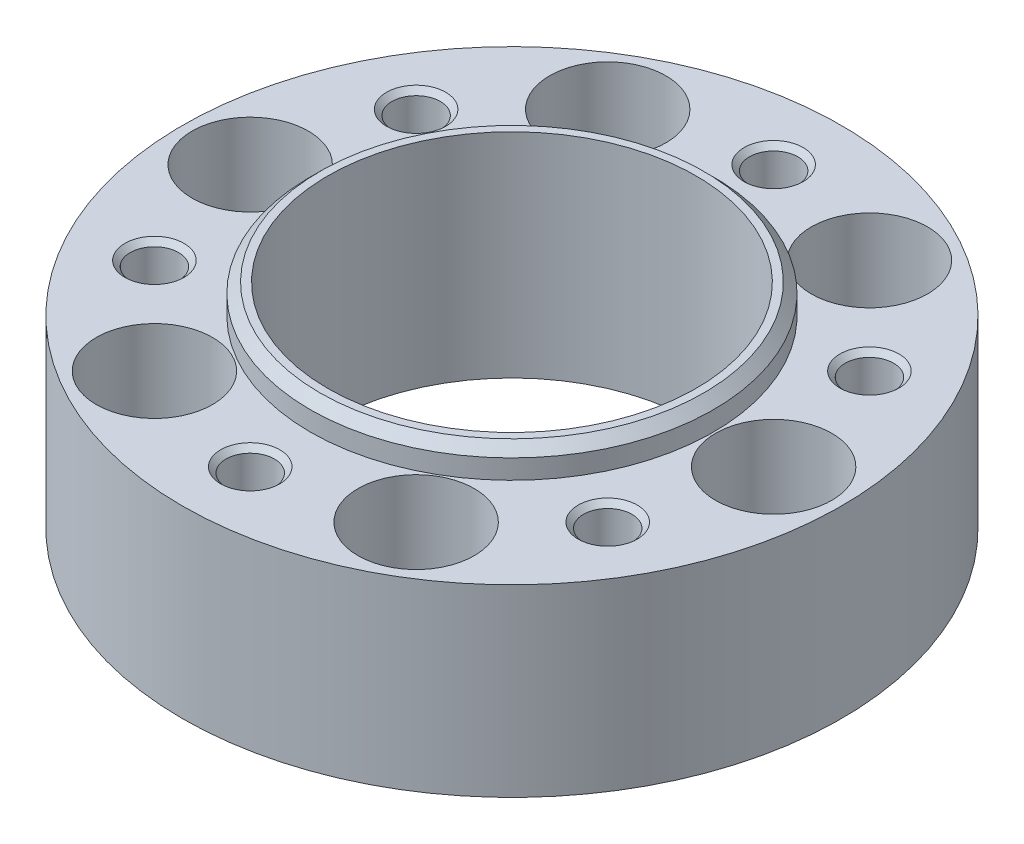
SolidWorks part; units mm, degrees
material "6061 合金"
ref_plane "前视基准面" through (0, 0, 0) normal (0, 0, 1) x (1, 0, 0)
ref_plane "上视基准面" through (0, 0, 0) normal (0, 1, 0) x (1, 0, 0)
ref_plane "右视基准面" through (0, 0, 0) normal (1, 0, 0) x (0, 0, -1)
other "Configuration Table"
sketch "草图1" plane through (0, 0, 0) normal (0, 1, 0) x (1, 0, 0)
  line L0 (0, 0) -> (23.0599, 0) construction
  line L1 (0, 0) -> (0, 21.1795) construction
  circle A0 centre (0, 0) radius 17
  circle A1 centre (0, 0) radius 13.5 construction
  circle A2 centre (13.5, 0) radius 1.55
  circle A3 centre (6.75, -11.6913) radius 1.55
  circle A4 centre (-6.75, -11.6913) radius 1.55
  circle A5 centre (-13.5, 0) radius 1.55
  circle A6 centre (-6.75, 11.6913) radius 1.55
  circle A7 centre (6.75, 11.6913) radius 1.55
  circle A8 centre (0, 0) radius 9.5
  point P21 (0, 0)
  dimension "D1" = 34
  dimension "D2" = 27
  dimension "D3" = 3.1
  dimension "D5" = 19
  dimension "D4" = 6
extrude "凸台-拉伸1" add sketch "草图1" along normal blind 9.5
sketch "草图2" plane through (0, 9.5, 0) normal (0, 1, 0) x (1, 0, 0)
  line L0 (0, 0) -> (21.6621, 0) construction
  line L1 (0, 0) -> (11.6913, 6.75) construction
  circle A0 centre (0, 0) radius 13.5 construction
  circle A1 centre (11.6913, 6.75) radius 0.5 construction
  circle A2 centre (11.6913, -6.75) radius 0.5 construction
  circle A3 centre (0, -13.5) radius 0.5 construction
  circle A4 centre (-11.6913, -6.75) radius 0.5 construction
  circle A5 centre (-11.6913, 6.75) radius 0.5 construction
  circle A6 centre (0, 13.5) radius 0.5 construction
  point P5 (11.6913, 6.75)
  point P11 (11.6913, -6.75)
  point P13 (0, -13.5)
  point P15 (-11.6913, -6.75)
  point P17 (-11.6913, 6.75)
  point P19 (0, 13.5)
  point P20 (0, 0)
  point P27 (11.6913, 6.75)
  dimension "D1" = 27
  dimension "D3" = 1
  dimension "D2" = 30
  dimension "D4" = 6
hole_wizard "M3 螺纹孔1" positions "草图2" profile "草图4" tap size "M3" standard "GB" end condition through all
sketch "草图4" plane through (11.6913, 9.5, -6.75) normal (1, 0, 0) x (0, 0, 1)
  line L0 (0, 0) -> (0, 9.5)
  line L1 (0, 9.5) -> (1.25, 9.5)
  line L2 (1.25, 9.5) -> (1.25, 0.275)
  line L3 (1.25, 0.275) -> (1.525, 0)
  line L5 (1.525, 0) -> (0, 0)
  line L6 (-1.25, 0.275) -> (-1.525, 0) construction
  line L11 (0, -6.35) -> (0, 107.95) construction
  dimension "通孔螺纹孔钻头直径" = 2.5
  dimension "通孔螺纹孔钻头深度" = 9.5
  dimension "近端锥形沉头孔直径" = 3.05
  dimension "近端锥形沉头孔角度" = 90
cosmetic thread "孔螺纹线1" parameters "D2"=3
cosmetic thread "孔螺纹线2" parameters "D2"=3
cosmetic thread "孔螺纹线3" parameters "D2"=3
cosmetic thread "孔螺纹线4" parameters "D2"=3
cosmetic thread "孔螺纹线5" parameters "D2"=3
cosmetic thread "孔螺纹线6" parameters "D2"=3
sketch "草图7" plane through (0, 9.5, 0) normal (0, 1, 0) x (1, 0, 0)
  circle A0 centre (0, 0) radius 10.4
  circle A1 centre (0, 0) radius 9.5 construction
  circle A2 centre (0, 0) radius 9.5
  dimension "D1" = 0.9
extrude "凸台-拉伸2" add sketch "草图7" along normal blind 1.5
sketch "草图5" plane through (0, 9.5, 0) normal (0, 1, 0) x (1, 0, 0)
  circle A0 centre (13.5, 0) radius 3
  circle A1 centre (6.75, -11.6913) radius 3
  circle A2 centre (-6.75, -11.6913) radius 3
  circle A3 centre (-13.5, 0) radius 3
  circle A4 centre (-6.75, 11.6913) radius 3
  circle A5 centre (6.75, 11.6913) radius 3
  point P15 (0, 0)
  dimension "D1" = 6
  dimension "D2" = 6
extrude "切除-拉伸1" cut sketch "草图5" against normal blind 5.5
chamfer "倒角1" distance 0.5 angle 45 1 edges at (0, 11, 10.4)
